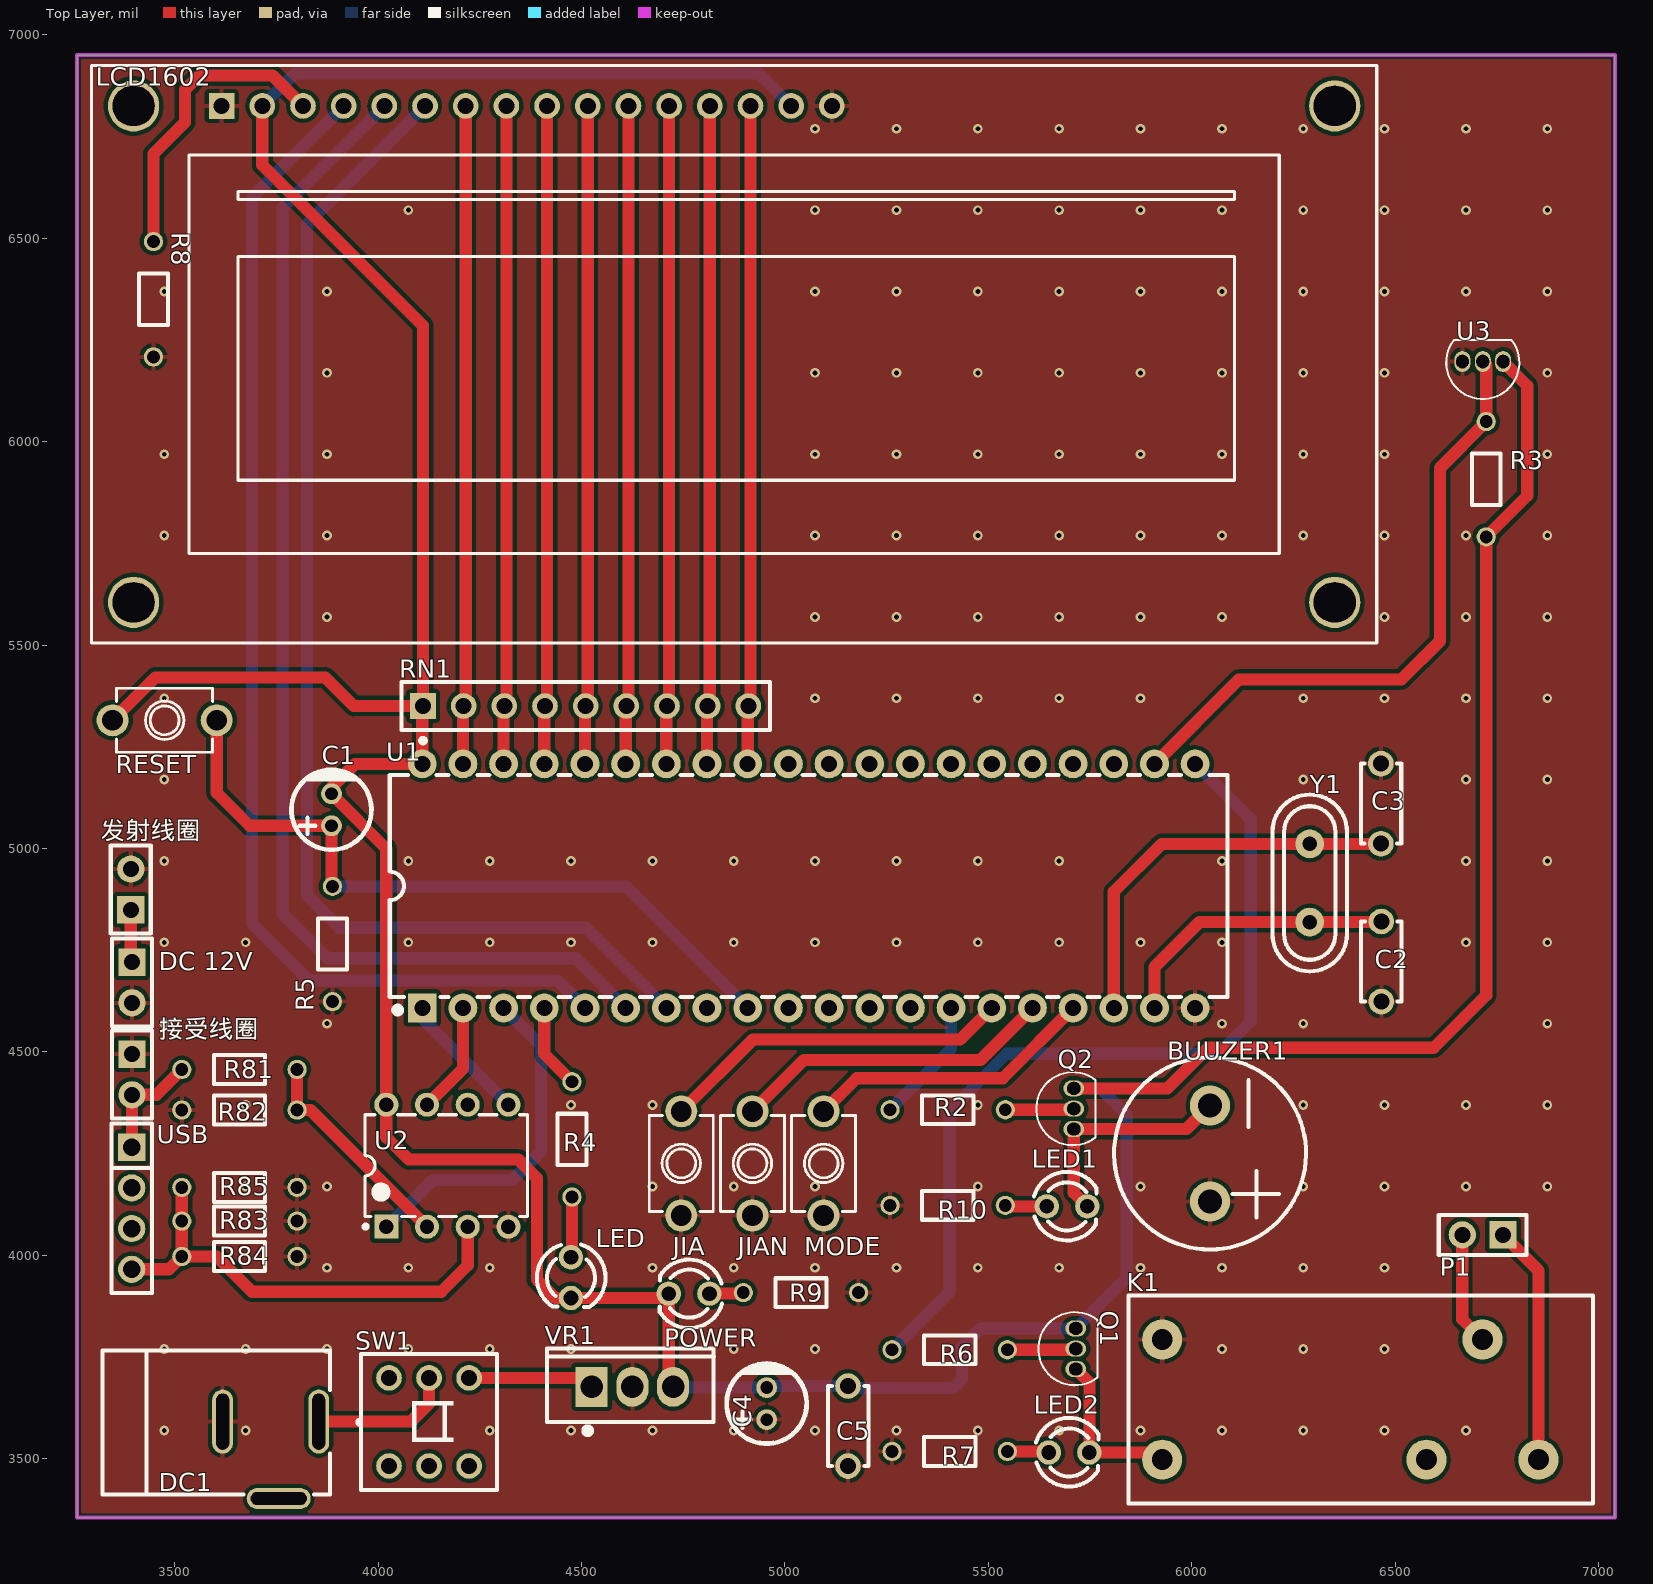
[diagram p0: Top Layer view]
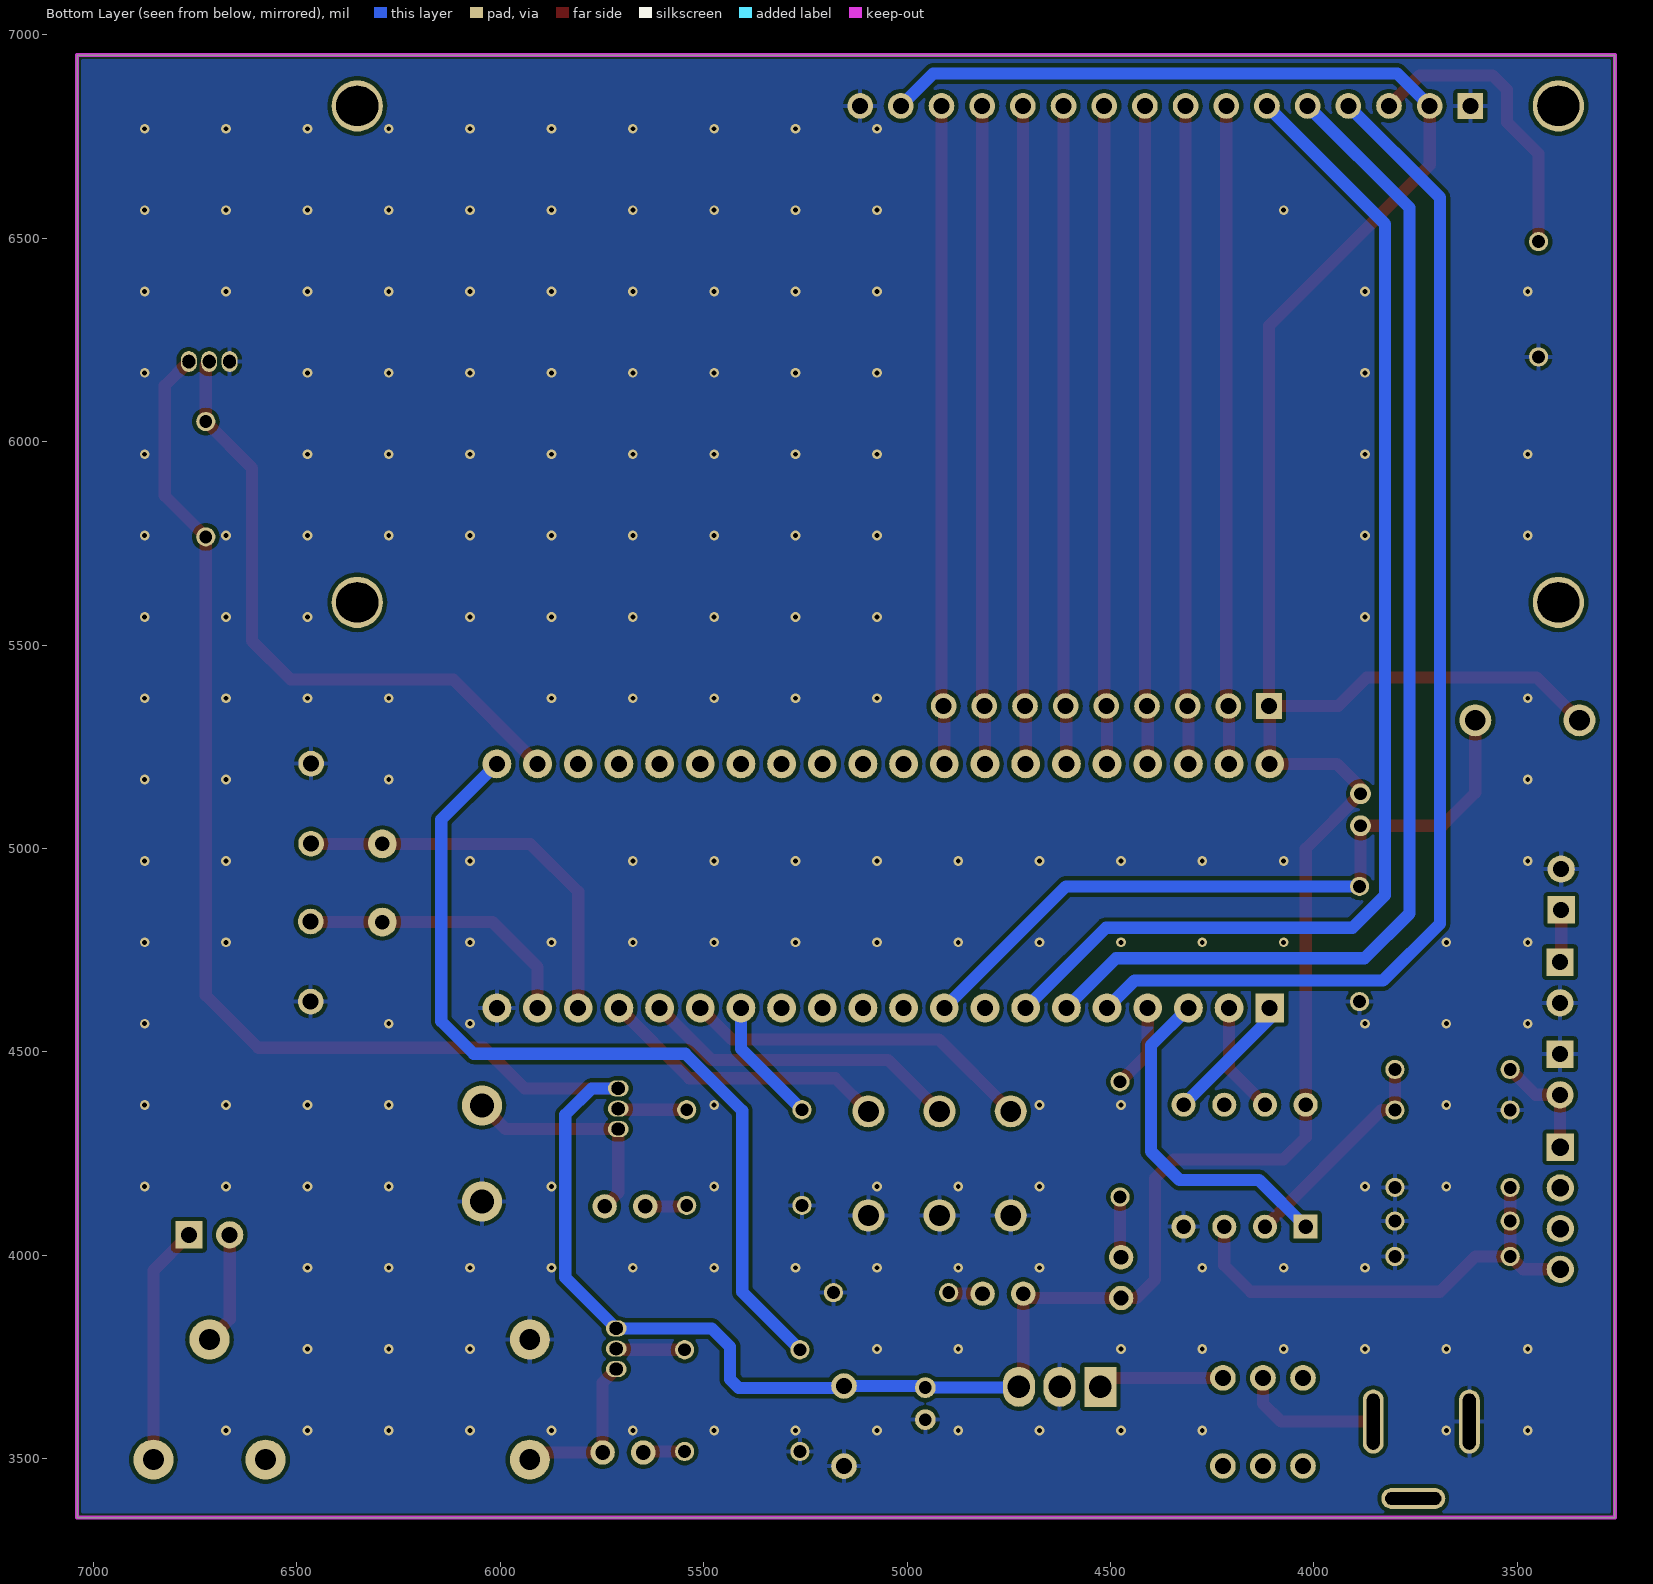
[diagram p1: Bottom Layer view, seen from below]
# Altium PCB MISC51120.pcbdoc
Units mil, origin at the board's own origin, x right, y up, seen from the top; angles counter-clockwise.
Board outline 3780 x 3595 mil, 2 copper layers (Top Layer, Bottom Layer), stack 62.206 mil thick; 45 components, 44 nets, 173 pads, 182 vias.

## Layer stack, top to bottom
Top Solder Mask Layer: solder mask 0.394, Dk 3.3
Top Layer: signal copper 1.379
Dielectric1: surface 59.449, FR4, Dk 4.5
Bottom Layer: signal copper 1.378
Bottom Solder Mask Layer: solder mask 0.394, Dk 3.3

## Board outline
3260,6950 3260,3355 7040,3355 7040,6950

## Design rules (kind name [scope] priority, off if disabled: settings)
BoardOutlineClearance copperThickness2oz_1 [All] p2 off: genericclearance=7.99 ignorepadtopadclearanceinfootprint=FALSE except(0: Arc-SplitContinuation Track-SplitContinuation SMDPad-SplitContinuation THPad-SplitContinuation Via-SplitContinuation Fill-SplitContinuation Region-SplitContinuation Poly-SplitContinuation Text-SplitContinuation Hole-SplitContinuation; 5.98: Arc-CutoutEdge SMDPad-CutoutEdge THPad-CutoutEdge Via-CutoutEdge Fill-CutoutEdge Region-CutoutEdge Text-CutoutEdge; 6.93: Hole-OutlineEdge Hole-CutoutEdge; 10: Poly-OutlineEdge Poly-CutoutEdge; 11.81: Arc-OutlineEdge Track-OutlineEdge SMDPad-OutlineEdge THPad-OutlineEdge Via-OutlineEdge Fill-OutlineEdge Region-OutlineEdge Text-OutlineEdge Track-CutoutEdge)
BoardOutlineClearance copperThickness1oz_1 [All] p4: genericclearance=4.02 ignorepadtopadclearanceinfootprint=FALSE except(0: Arc-SplitContinuation Track-SplitContinuation SMDPad-SplitContinuation THPad-SplitContinuation Via-SplitContinuation Fill-SplitContinuation Region-SplitContinuation Poly-SplitContinuation Text-SplitContinuation Hole-SplitContinuation; 6: SMDPad-CutoutEdge THPad-CutoutEdge Via-CutoutEdge Fill-CutoutEdge Region-CutoutEdge Text-CutoutEdge; 6.93: Hole-OutlineEdge Hole-CutoutEdge; 10: Poly-OutlineEdge Poly-CutoutEdge; 11.8: Arc-OutlineEdge Track-OutlineEdge SMDPad-OutlineEdge THPad-OutlineEdge Via-OutlineEdge Fill-OutlineEdge Region-OutlineEdge Text-OutlineEdge; 11.81: Arc-CutoutEdge Track-CutoutEdge)
Clearance copperThickness2oz [All] p1 off: gap=7.99 ignorepadtopadclearanceinfootprint=FALSE except(5.98: SMDPad-Track SMDPad-SMDPad THPad-Track SMDPad-THPad THPad-THPad Track-Via SMDPad-Via THPad-Via Via-Via Fill-Track Region-Track Fill-SMDPad Region-SMDPad Fill-THPad Region-THPad Fill-Via Region-Via Fill-Fill Fill-Region Region-Region Arc-Track Arc-SMDPad Arc-THPad Arc-Via Fill-Arc Region-Arc Arc-Arc Text-Track SMDPad-Text Text-THPad Text-Via Fill-Text Region-Text Arc-Text Text-Text; 6.93: Hole-Track Hole-SMDPad Hole-THPad Hole-Via Fill-Hole Region-Hole Hole-Arc Hole-Text; 10: Poly-Track Poly-SMDPad Poly-THPad Poly-Via Poly-Fill Poly-Region Poly-Poly Poly-Arc Poly-Text Poly-Hole)
Clearance copperThickness1oz [All] p3: gap=4.02 ignorepadtopadclearanceinfootprint=FALSE except(5.98: SMDPad-Track SMDPad-SMDPad THPad-Track SMDPad-THPad THPad-THPad Track-Via SMDPad-Via THPad-Via Via-Via Fill-Track Region-Track Fill-SMDPad Region-SMDPad Fill-THPad Region-THPad Fill-Via Region-Via Fill-Fill Fill-Region Region-Region; 6: Arc-Track Arc-SMDPad Arc-THPad Arc-Via Fill-Arc Region-Arc Arc-Arc Text-Track SMDPad-Text Text-THPad Text-Via Fill-Text Region-Text Arc-Text Text-Text; 6.93: Hole-Track Hole-SMDPad Hole-THPad Hole-Via Fill-Hole Region-Hole Hole-Arc Hole-Text; 10: Poly-Track Poly-SMDPad Poly-THPad Poly-Via Poly-Fill Poly-Region Poly-Poly Poly-Arc Poly-Text Poly-Hole)
Creepage creepage [All] p1: checkdistance=0 ignoreinternallayers=TRUE applytopolygonpour=TRUE
DiffPairsRouting differentialPair [All] p1: maxlimit=6 minlimit=6 mostfreqgap=6 toplayer_minwidth=5 toplayer_prefwidth=10 toplayer_maxwidth=100 toplayer_mingap=6 toplayer_prefgap=6 toplayer_maxgap=6 bottomlayer_minwidth=5 bottomlayer_prefwidth=10 bottomlayer_maxwidth=100 bottomlayer_mingap=6 bottomlayer_prefgap=6 bottomlayer_maxgap=6 maxuncoupledlength=10
HoleToHoleClearance otherClearance [All] p1: gap=11.81 allowstackedmicrovias=TRUE
Length netLength [All] p1: minlimit=0 maxlimit=0
MatchedLengths netLengthTolerance [All] p1: tolerance=1000
PasteMaskExpansion pasteMaskExpansion [All] p1: expansion=0
PlaneConnect innerPlane [All] p1: planeconnectstyle=Relief reliefexpansion=20 reliefentries=4 reliefconductorwidth=10 reliefairgap=10
PolygonConnect copperRegion [(InNet('GND'))] p1: connectstyle=Relief reliefconductorwidth=10 reliefentries=4 polygonreliefangle="90 Angle" airgapwidth=10 via.connectstyle=Relief via.reliefconductorwidth=10 via.reliefentries=4 via.polygonreliefangle="90 Angle" via.airgapwidth=10
RoutingVias viaSize [All] p1: holewidth=12.01 width=24.02 viastyle="Through Hole" minholewidth=11.81 minwidth=19.68 maxholewidth=248.03 maxwidth=393.7
SolderMaskExpansion solderMaskExpansion [IsVia] p1: expansion=-1000 istentingtop=TRUE
SolderMaskExpansion solderMaskExpansion [All] p2: expansion=2 istentingtop=FALSE
Width copperThickness2oz_2 [All] p1 off: maxlimit=100 minlimit=8 preferedwidth=10
Width copperThickness1oz_2 [All] p2: maxlimit=100 minlimit=5 preferedwidth=10

## Components (designator, comment, footprint, x,y, rotation, side; value= is the part's Value field where it differs from the comment)
BUUZER1 "BUZZER" BUZ-TH_BD12.0-P6.00-D0.9-RD 6045,4250 r270 top
C1 "10uF" CAP-TH_BD5.0-P2.00-D0.8-FD-10UF50VC110GL 3885,5095 r90 top
C2 "18pF" CAP-TH_L5.0-W2.5-P5.00-D1.0 6465.98,4721.82 r270 top
C3 "18pF" CAP-TH_L5.0-W2.5-P5.00-D1.0 6465,5110 r90 top
C4 "470uF" CAP-TH_BD5.0-P2.00-D0.8-FD-10UF50VC110GL 4955,3635 r90 top
C5 "104" CAP-TH_L5.0-W2.5-P5.00-D1.0 5155,3580 r90 top
DC1 "" DC-2.0 3730.7,3601.37 r180 top
"DC 12V" "Header 2" HDR-TH_2P-P2.54-V-F 3394.7,4670.39 r270 top
JIA "SW-PB" KEY-TH_2P-L6.0-W3.9-P6.50 4745,4225.64 r90 top
JIAN "SW-PB" KEY-TH_2P-L6.0-W3.9-P6.50 4920,4225.64 r90 top
K1 "继电器" RELAY-TH_G2R-1_C9900014679 6390,3645 r0 top
LCD1602 "LCD1602" LCD1602 4875,6215 r0 top
LED "SI3317-H" LED_TH-3mm 4473.82,3944.7 r270 top
LED1 "SI3317-H" LED_TH-3mm 5693.41,4120 r0 top
LED2 "SI3317-H" LED_TH-3mm 5698.41,3515 r0 top
MODE "SW-PB" KEY-TH_2P-L6.0-W3.9-P6.50 5095,4225.64 r90 top
P1 "Header 2" HDR-TH_2P-P2.54-V-F 6715,4050 r180 top
POWER "SI3317-H" LED_TH-3mm 4764.26,3905.44 r180 top
Q1 "S8550" TO-92-3_L4.6-W3.6-P1.27-L_1 5715,3770 r270 top
Q2 "S8550" TO-92-3_L4.6-W3.6-P1.27-L_1 5710,4360 r270 top
R2 "470" Res_1/8W 5400,4360 r180 top
R3 "10K" Res_1/8W 6721.33,5907.6 r270 top
R4 "470" Res_1/8W 4473.82,4284.7 r270 top
R5 "10K" Res_1/8W 3890,4765 r90 top
R6 "470" Res_1/8W 5405,3770 r180 top
R7 "470" Res_1/8W 5405,3515 r0 top
R8 "470" Res_1/8W 3445,6350 r270 top
R9 "470" Res_1/8W 5039.26,3910.44 r180 top
R10 "470" Res_1/8W 5400,4120 r0 top
R81 "470" Res_1/8W 3658.91,4454.16 r0 top
R82 "470" Res_1/8W 3658.91,4359.16 r180 top
R83 "470" Res_1/8W 3658.91,4081.3 r0 top
R84 "470" Res_1/8W 3658.91,3994.21 r0 top
R85 "470" Res_1/8W 3658.91,4164.16 r0 top
RESET "SW-PB" KEY-TH_2P-L6.0-W3.9-P6.50 3475,5315 r180 top
RN1 "-" RES-ARRAY-TH_9P-P2.54-D1.0 4510,5350 r0 top
SW1 "sw-灰色" SW-TH_6P-L8.5-W8.5-P2.54 4125,3590 r0 top
U1 "STC89C52" DIP-40_L52.3-W13.9-P2.54-LS15.2-BL-BASE 5058.32,4907.72 r0 top
U2 "ADC0832" DIP-8_L10.1-W6.3-P2.54-LS7.6-BL 4170,4220 r0 top
U3 "DS18B20" TO-92-3_L4.6-W3.6-P1.27-L_1 6715.47,6196.79 r0 top
USB "Header 4" HDR-TH_4P-P2.54-V-F 3393.91,4115.39 r270 top
VR1 "L7805" TO-220AB-3_L10.4-W4.6-P2.54-L 4624.87,3676.37 r0 top
Y1 "11.0592M" HC-49S_L11.0-W4.7-P4.88 6290,4915 r270 top
发射线圈 "Header 2" HDR-TH_2P-P2.54-V-F 3391.67,4899.16 r90 top
接受线圈 "Header 2" HDR-TH_2P-P2.54-V-F 3394.7,4444.16 r270 top

## Footprints (in the part's own frame and the unit in brackets; to place one, negate y for a bottom-side part, rotate by r counter-clockwise, add the part's x,y. Pads: shape width x height; smd on the part's side, far side on the other; paste and mask are expansions set on the pad)
BUZ-TH_BD12.0-P6.00-D0.9-RD [mm]
  round 2.5 hole 1.5 paste+0 mask+0.05: 1(-3,0) 2(3,0)
  silkscreen extent -5.99,-5.99 5.99,5.99
CAP-TH_BD5.0-P2.00-D0.8-FD-10UF50VC110GL [mm]
  round 1.3 hole 0.8: 1(-1,0) 2(1,0)
  silkscreen extent -2.5,-2.5 2.5,2.5
CAP-TH_L5.0-W2.5-P5.00-D1.0 [mm]
  round 1.6 hole 1: 1(-2.5,0) 2(2.5,0)
  silkscreen extent -2.5,-1.27 2.5,1.25
DC-2.0 [mil]
  oval 157.5x51.2 hole 31.5 slot 137.8 at 0 deg paste+0 mask+2: 2(-24.7,199.5)
  oval 51.2x157.5 hole 31.5 slot 137.8 at 90 deg paste+0 mask+2: 3(113.1,10.5) 4(-123.1,10.5)
  silkscreen extent -151,-165 408,190
DIP-8_L10.1-W6.3-P2.54-LS7.6-BL [mm]
  rect 1.5x1.5 hole 0.9: 1(-3.81,-3.81)
  round 1.5 hole 0.9: 2(-1.27,-3.81) 3(1.27,-3.81) 4(3.81,-3.81) 5(3.81,3.81) 6(1.27,3.81) 7(-1.27,3.81) 8(-3.81,3.81)
  silkscreen extent -5.23,-3.93 5.01,3.17
DIP-40_L52.3-W13.9-P2.54-LS15.2-BL-BASE [mm]
  rect 1.8x1.8 hole 1: 1(-24.13,-7.62)
  round 1.8 hole 1: 2(-21.59,-7.62) 3(-19.05,-7.62) 4(-16.51,-7.62) 5(-13.97,-7.62) 6(-11.43,-7.62) 7(-8.89,-7.62) 8(-6.35,-7.62) 9(-3.81,-7.62) 10(-1.27,-7.62) 11(1.27,-7.62) 12(3.81,-7.62) 13(6.35,-7.62) 14(8.89,-7.62) 15(11.43,-7.62) 16(13.97,-7.62) 17(16.51,-7.62) 18(19.05,-7.62) 19(21.59,-7.62) 20(24.13,-7.62) 21(24.13,7.62) 22(21.59,7.62) 23(19.05,7.62) 24(16.51,7.62) 25(13.97,7.62) 26(11.43,7.62) 27(8.89,7.62) 28(6.35,7.62) 29(3.81,7.62) 30(1.27,7.62) 31(-1.27,7.62) 32(-3.81,7.62) 33(-6.35,7.62) 34(-8.89,7.62) 35(-11.43,7.62) 36(-13.97,7.62) 37(-16.51,7.62) 38(-19.05,7.62) 39(-21.59,7.62) 40(-24.13,7.62)
  silkscreen extent -26.16,-7.95 26.16,6.93
HC-49S_L11.0-W4.7-P4.88 [mm]
  round 1.8 hole 0.9: 1(-2.44,0) 2(2.44,0)
  silkscreen extent -5.52,-2.32 5.52,2.33
HDR-TH_2P-P2.54-V-F [mm]
  rect 1.7x1.7 hole 1: 1(-1.27,0)
  round 1.7 hole 1: 2(1.27,0)
  silkscreen extent -2.74,-1.25 2.74,1.25
HDR-TH_4P-P2.54-V-F [mm]
  rect 1.7x1.7 hole 1.1: 1(-3.81,0)
  round 1.7 hole 1.1: 2(-1.27,0) 3(1.27,0) 4(3.81,0)
  silkscreen extent -5.29,-1.27 5.29,1.27
KEY-TH_2P-L6.0-W3.9-P6.50 [mm]
  round 2 hole 1.3: 1(-3.25,0) 2(3.25,0)
  silkscreen extent -3,-2 3,2
LCD1602 [mm]
  round 3.2 hole 2.5 slot 2.625 at 0 deg: 0(-37.5,-15.5) 0(-37.5,15.5) 0(37.5,-15.5) 0(37.5,15.5)
  rect 1.6x1.6 hole 1: 1(-32,15.5)
  round 1.6 hole 1: 2(-29.46,15.5) 3(-26.92,15.5) 4(-24.38,15.5) 5(-21.84,15.5) 6(-19.3,15.5) 7(-16.76,15.5) 8(-14.22,15.5) 9(-11.68,15.5) 10(-9.14,15.5) 11(-6.6,15.5) 12(-4.06,15.5) 13(-1.52,15.5) 14(1.02,15.5) 15(3.56,15.5) 16(6.1,15.5)
  silkscreen extent -40.13,-18.03 40.13,18.03
LED_TH-3mm [mil]
  round 60 hole 36 paste+0 mask+2: 1(-50,0) 2(50,0)
  silkscreen extent -81,-84 72,85
RELAY-TH_G2R-1_C9900014679 [mm]
  round 2.5 hole 1.3 paste+0 mask+0.05: 1(-11.75,-3.75) 2(4.75,-3.75) 3(11.75,-3.75) 4(8.25,3.75) 5(-11.75,3.75)
  silkscreen extent -13.85,-6.5 15.15,6.5
RES-ARRAY-TH_9P-P2.54-D1.0 [mm]
  rect 1.6x1.6 hole 1: 1(-10.16,0)
  round 1.6 hole 1: 2(-7.62,0) 3(-5.08,0) 4(-2.54,0) 5(0,0) 6(2.54,0) 7(5.08,0) 8(7.62,0) 9(10.16,0)
  silkscreen extent -11.5,-2.31 11.5,1.5
Res_1/8W [mil]
  round 47.2 hole 31.5 paste+0 mask+2: 1(-141.7,2.48) 2(141.7,2.48)
  silkscreen extent -63,-33 63,38
SW-TH_6P-L8.5-W8.5-P2.54 [mm]
  round 1.6 hole 1: 1(-2.5,-2.75) 2(0,-2.75) 3(2.5,-2.75) 4(-2.5,2.75) 5(0,2.75) 6(2.5,2.75)
  silkscreen extent -4.47,-4.25 4.25,4.25
TO-92-3_L4.6-W3.6-P1.27-L_1 [mm]
  oval 1x1.3 hole 0.8 slot 0.84 at 90 deg paste+0 mask+0.05: 1(-1.27,0) 2(0,0) 3(1.27,0)
  silkscreen extent -2.28,-2.34 2.28,1.35
TO-220AB-3_L10.4-W4.6-P2.54-L [mm]
  rect 2x2.5 hole 1.4: 1(-2.54,0)
  oval 2x2.5 hole 1.4: 2(0,0) 3(2.54,0)
  silkscreen extent -5.33,-2.94 5.08,2.4

## Via types
v1: diameter 24.02, hole 12, Top Layer to Bottom Layer, 182 vias

## Nets (pads, with @x,y where several pads share a name; then routed paths per layer and width w, separated by ;. In a path a pad name is that pad's centre, name@x,y a point inside that pad or via, vN(x,y) a via of type N, cw(c..) or ccw(c..) an arc to the next point about the centre after c; other vN are vias at no path point)
$2N76: BUUZER1.1 LED1.2 Q2.3 | length 562.9
  Top Layer w30: LED1.2 5710,4153.41 Q2.3 5986.89,4310 BUUZER1.1
$2N77: LED1.1 R10.2 | length 102.7
  Top Layer w30: R10.2 5544.18,4120 LED1.1
$2N78: Q2.2 R2.1 | length 169.3
  Top Layer w30: R2.1 5707.52,4357.52 Q2.2
$2N79: Q1.2 R6.1 | length 169.3
  Top Layer w30: R6.1 5712.52,3767.52 Q1.2
$2N80: LED.1 R4.2 | length 149.3
  Top Layer w30: LED.1 4476.29,3997.18 R4.2
$2N81: POWER.1 R9.2 | length 84.3
  Top Layer w30: POWER.1 4895.03,3905.44 R9.2
$2N114: "DC 12V.1" 发射线圈.1 | length 130
  Top Layer w30: 发射线圈.1 3391.67,4723.42 3394.7,4720.39
$2N115: K1.3 P1.1 | length 588.9
  Top Layer w30: P1.1 6852.6,3962.4 K1.3
$2N116: K1.4 P1.2 | length 278
  Top Layer w30: P1.2 6665,3842.44 K1.4
$2N126: K1.1 LED2.2 Q1.3 | length 405.1
  Top Layer w30: Q1.3 5748.41,3686.59 LED2.2 5909.77,3515 K1.1
$2N127: LED2.1 R7.2 | length 102.7
  Top Layer w30: R7.2 5645.93,3517.48 LED2.1
$2N133: SW1.6 VR1.1 | length 310.5
  Top Layer w30: SW1.6 4502.97,3698.27 VR1.1
$2N134: DC1.4 SW1.5 | length 352.7
  Top Layer w30: DC1.4 4080.87,3590.87 4124.99,3634.99 SW1.5
$2N139: R81.1 USB.1 接受线圈.2 | length 277.5
  Top Layer w30: USB.1 3394.7,4266.18 接受线圈.2 3454.74,4394.16 R81.1
$2N149: LCD1602.3 R8.1 | length 741
  Top Layer w30: R8.1 3447.48,6707.48 3525,6785 3525,6865 3560,6900 3740.4,6900 LCD1602.3
BUZZER: R2.2 U1.14 | length 312.3
  Bottom Layer w30: R2.2 5408.32,4507.54 U1.14
CH0: R81.2 R82.1 U2.2 | length 538.1
  Top Layer w30: R81.2 R82.1 3833.32,4356.68 U2.2
CH1: R83.1 R84.1 R85.1 U2.3 USB.4 | length 1166.8
  Top Layer w30: USB.4 3485.92,3965.39 R84.1 ; R85.1 R83.1 R84.1 ; U2.3 4220,3975 4155,3910 3690,3910 3603.32,3996.68 R84.1
CLK: U1.2 U2.7 | length 274.3
  Top Layer w30: U2.7 4208.32,4458.32 U1.2
CS: U1.3 U2.1 | length 847.3
  Bottom Layer w30: U2.1 4135,4185 4330,4185 4400,4255 4400,4516.03 U1.3
DATA: R3.1 U1.22 U3.2 | length 1564.3
  Top Layer w30: U1.22 6115.6,5415 6515,5415 6610,5510 6610,5935.49 R3.1 6723.81,6188.45 U3.2
DB0: LCD1602.7 RN1.2 U1.39 | length 1607.5
  Top Layer w30: U1.39 RN1.2@4208.32,5350 ; RN1.2@4215.16,5360 LCD1602.7
DB1: LCD1602.8 RN1.3 U1.38 | length 1607.5
  Top Layer w30: U1.38 RN1.3@4308.32,5350 ; RN1.3@4315.16,5360 LCD1602.8
DB2: LCD1602.9 RN1.4 U1.37 | length 1607.5
  Top Layer w30: U1.37 RN1.4@4408.32,5350 ; RN1.4@4415.16,5360 LCD1602.9
DB3: LCD1602.10 RN1.5 U1.36 | length 1607.5
  Top Layer w30: U1.36 RN1.5@4508.32,5350 ; RN1.5@4515.16,5360 LCD1602.10
DB4: LCD1602.11 RN1.6 U1.35 | length 1607.5
  Top Layer w30: U1.35 RN1.6@4608.32,5350 ; RN1.6@4615.16,5360 LCD1602.11
DB5: LCD1602.12 RN1.7 U1.34 | length 1607.5
  Top Layer w30: U1.34 RN1.7@4708.32,5350 ; RN1.7@4715.16,5360 LCD1602.12
DB6: LCD1602.13 RN1.8 U1.33 | length 1607.5
  Top Layer w30: U1.33 RN1.8@4808.32,5350 ; RN1.8@4815.16,5360 LCD1602.13
DB7: LCD1602.14 RN1.9 U1.32 | length 1607.5
  Top Layer w30: U1.32 RN1.9@4908.32,5350 ; RN1.9@4915.16,5360 LCD1602.14
DI: U1.1 U2.5 | length 325.4
  Bottom Layer w30: U1.1 4108.32,4581.68 U2.5
DO: U2.6
EN: LCD1602.6 U1.7 | length 3058.6
  Bottom Layer w30: LCD1602.6 3825,6535.08 3825,4885 3905,4805 4511.03,4805 U1.7
GND: "DC 12V.2" BUUZER1.2 C2.2 C3.2 C4.1 C5.1 DC1.3 JIA.1 JIAN.1 K1.5 LCD1602.1 LCD1602.16 MODE.1 R5.1 R7.1 R8.2 R9.1 R10.1 R82.2 R83.2 R84.2 R85.2 U1.20 U2.4 U3.1 VR1.2 发射线圈.2 接受线圈.1
  other v1: 3474.1,3569.1 3674.1,3569.1 4274.1,3569.1 4474.1,3569.1 4674.1,3569.1 4874.1,3569.1 5074.1,3569.1 5274.1,3569.1 5474.1,3569.1 5674.1,3569.1 5874.1,3569.1 6074.1,3569.1 6274.1,3569.1 6474.1,3569.1 6674.1,3569.1 3474.1,3769.1 3674.1,3769.1 3874.1,3769.1 4074.1,3769.1 4274.1,3769.1 4474.1,3769.1 4874.1,3769.1 5074.1,3769.1 6074.1,3769.1 6274.1,3769.1 6474.1,3769.1 3874.1,3969.1 4074.1,3969.1 4274.1,3969.1 4674.1,3969.1 4874.1,3969.1 5074.1,3969.1 5274.1,3969.1 5474.1,3969.1 5674.1,3969.1 5874.1,3969.1 6074.1,3969.1 6274.1,3969.1 6474.1,3969.1 3674.1,4169.1 3874.1,4169.1 4674.1,4169.1 4874.1,4169.1 5074.1,4169.1 5474.1,4169.1 5874.1,4169.1 6274.1,4169.1 6474.1,4169.1 6674.1,4169.1 6874.1,4169.1 3674.1,4369.1 4474.1,4369.1 4674.1,4369.1 5474.1,4369.1 6274.1,4369.1 6474.1,4369.1 6674.1,4369.1 6874.1,4369.1 3474.1,4569.1 3674.1,4569.1 3874.1,4569.1 6074.1,4569.1 6274.1,4569.1 6874.1,4569.1 3474.1,4769.1 3674.1,4769.1 4074.1,4769.1 4274.1,4769.1 4474.1,4769.1 4674.1,4769.1 4874.1,4769.1 5074.1,4769.1 5274.1,4769.1 5474.1,4769.1 5674.1,4769.1 5874.1,4769.1 6074.1,4769.1 6674.1,4769.1 6874.1,4769.1 3474.1,4969.1 4074.1,4969.1 4274.1,4969.1 4474.1,4969.1 4674.1,4969.1 4874.1,4969.1 5074.1,4969.1 5274.1,4969.1 5474.1,4969.1 5674.1,4969.1 6074.1,4969.1 6674.1,4969.1 6874.1,4969.1 3474.1,5169.1 6274.1,5169.1 6674.1,5169.1 6874.1,5169.1 3474.1,5369.1 5074.1,5369.1 5274.1,5369.1 5474.1,5369.1 5674.1,5369.1 5874.1,5369.1 6274.1,5369.1 6474.1,5369.1 6674.1,5369.1 6874.1,5369.1 3874.1,5569.1 5074.1,5569.1 5274.1,5569.1 5474.1,5569.1 5674.1,5569.1 5874.1,5569.1 6074.1,5569.1 6474.1,5569.1 6674.1,5569.1 6874.1,5569.1 3474.1,5769.1 3874.1,5769.1 5074.1,5769.1 5274.1,5769.1 5474.1,5769.1 5674.1,5769.1 5874.1,5769.1 6074.1,5769.1 6274.1,5769.1 6474.1,5769.1 6674.1,5769.1 6874.1,5769.1 3474.1,5969.1 3874.1,5969.1 5074.1,5969.1 5274.1,5969.1 5474.1,5969.1 5674.1,5969.1 5874.1,5969.1 6074.1,5969.1 6274.1,5969.1 6474.1,5969.1 6874.1,5969.1 3874.1,6169.1 5074.1,6169.1 5274.1,6169.1 5474.1,6169.1 5674.1,6169.1 5874.1,6169.1 6074.1,6169.1 6274.1,6169.1 6474.1,6169.1 6874.1,6169.1 3474.1,6369.1 3874.1,6369.1 5074.1,6369.1 5274.1,6369.1 5474.1,6369.1 5674.1,6369.1 5874.1,6369.1 6074.1,6369.1 6274.1,6369.1 6474.1,6369.1 6674.1,6369.1 6874.1,6369.1 4074.1,6569.1 5074.1,6569.1 5274.1,6569.1 5474.1,6569.1 5674.1,6569.1 5874.1,6569.1 6074.1,6569.1 6274.1,6569.1 6474.1,6569.1 6674.1,6569.1 6874.1,6569.1 5074.1,6769.1 5274.1,6769.1 5474.1,6769.1 5674.1,6769.1 5874.1,6769.1 6074.1,6769.1 6274.1,6769.1 6474.1,6769.1 6674.1,6769.1 6874.1,6769.1
K1: R6.2 U1.21 | length 2166.6
  Bottom Layer w30: R6.2 5405,3909.22 5405,4355 5545,4495 6065,4495 6145,4575 6145,5071.03 U1.21
KEY1: JIA.2 U1.15 | length 868.6
  Top Layer w30: JIA.2 4921.41,4530 5430.6,4530 U1.15
KEY2: JIAN.2 U1.16 | length 793.6
  Top Layer w30: JIAN.2 5046.41,4480 5480.6,4480 U1.16
KEY3: MODE.2 U1.17 | length 718.6
  Top Layer w30: MODE.2 5176.41,4435 5535.6,4435 U1.17
LED: R4.1 U1.4 | length 209.5
  Top Layer w30: U1.4 4408.32,4494.37 R4.1
RESET: C1.1 R5.2 RESET.1 U1.9 | length 1788.3
  Top Layer w30: RESET.1 3602.95,5137.05 3684.37,5055.63 C1.1 3885,4909.22 R5.2
  Bottom Layer w30: R5.2 4609.33,4906.7 U1.9
RS: LCD1602.4 U1.5 | length 3007.7
  Bottom Layer w30: LCD1602.4 3690,6600.08 3690,4815 3830,4675 4441.03,4675 U1.5
RW: LCD1602.5 U1.6 | length 3028.4
  Bottom Layer w30: LCD1602.5 3765,6575.08 3765,4840 3875,4730 4486.03,4730 U1.6
VCC: C1.2 C4.2 C5.2 LCD1602.2 LCD1602.15 LED.2 POWER.2 Q1.1 Q2.1 R3.2 RESET.2 RN1.1 U1.40 U2.8 U3.3 VR1.3 | length 10956.9
  Top Layer w30: RESET.2 3452.05,5420 3870,5420 3940,5350 RN1.1@4108.32,5350 ; LCD1602.2 3715.16,6679.84 4110,6285 RN1.1 RN1.1@4108.32,5350 ; VR1.3 4714.26,3686.99 POWER.2 4703.52,3894.7 LED.2 4435.3,3894.7 4390,3940 4390,4190 4345,4235 4075,4235 4020,4290 U2.8 4020,4999.37 C1.2 3885,5150 3942.72,5207.72 U1.40 RN1.1@4108.32,5350 ; Q2.1 5940,4410 6040,4510 6595,4510 6723.81,4638.81 R3.2 6825,5867.09 6825,6137.26 U3.3
  Bottom Layer w30: LCD1602.2 3794.92,6905 4935.4,6905 LCD1602.15 ; VR1.3 4726.87,3674.37 C4.2 4959.06,3678.43 C5.2 5159.64,3673.79 5413.79,3673.79 5435,3695 5435,3775 5480,3820 Q1.1 5840,3945 5840,4345 5775,4410 Q2.1
X1: C2.1 U1.19 Y1.2 | length 704.6
  Top Layer w30: U1.19 5908.32,4708.32 6018.94,4818.94 Y1.2 6464.67,4818.94 C2.1
X2: C3.1 U1.18 Y1.1 | length 991.3
  Top Layer w30: U1.18 5808.32,4893.32 5926.06,5011.06 Y1.1 6464.49,5011.06 C3.1
pads on no net: DC1.2 K1.2 LCD1602.0 SW1.1 SW1.2 SW1.3 SW1.4 U1.8 U1.10 U1.11 U1.12 U1.13 U1.23 U1.24 U1.25 U1.26 U1.27 U1.28 U1.29 U1.30 U1.31 USB.2 USB.3

## Polygon pours and split planes (outlines as drawn)
GND on Bottom Layer (solid, remove dead copper, pour order 2): 3000,7100 3000,3000 7305,3000 7305,7100
GND on Top Layer (solid, remove dead copper, pour order 0): 3055,7085 3055,3065 7210,3065 7210,7085

## Keep-outs
Board Outline Layer:
  the board outline again, w10